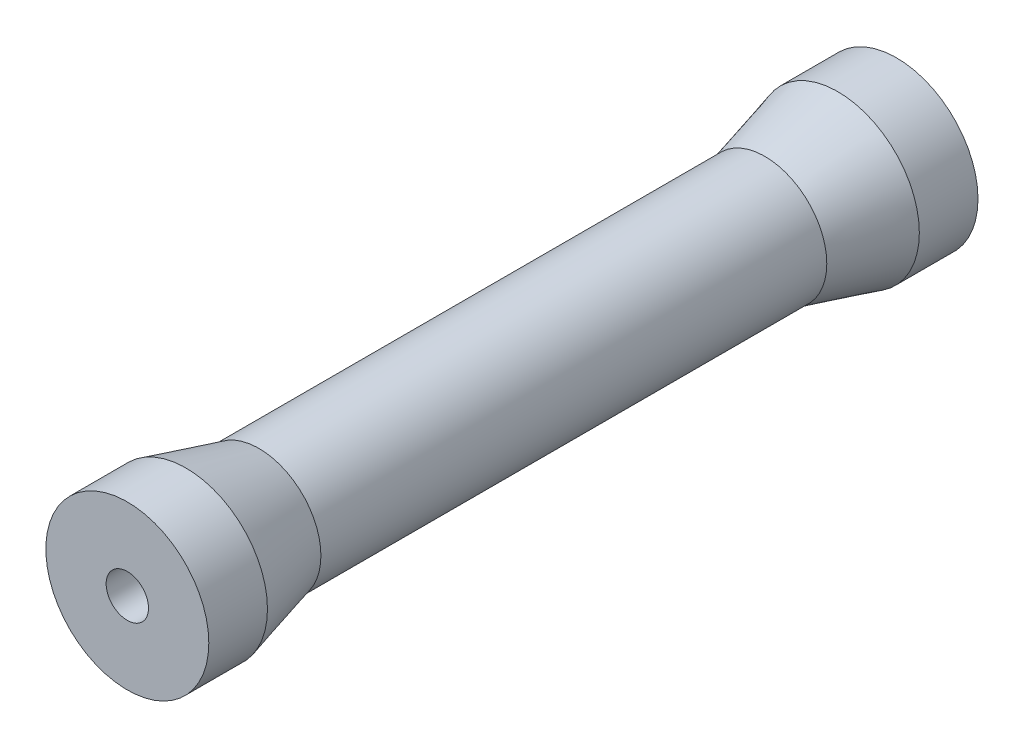
from build123d import *

# Parameters (mm, degrees)
SKETCH1_R           = 12.5
SKETCH1_R_2         = 3.25
BOSS_EXTRUDE1_DEPTH = 59


with BuildPart() as part:
    # Sketch1 → Boss-Extrude1 (new, symmetric)
    with BuildSketch(Plane.XY):
        Circle(SKETCH1_R)
        Circle(SKETCH1_R_2, mode=Mode.SUBTRACT)
    extrude(amount=BOSS_EXTRUDE1_DEPTH, both=True)

    # Sketch3 → Cut-Revolve1 (revolve, cut)
    with BuildSketch(Plane(origin=(0, 0, 0), x_dir=(1, 0, 0), z_dir=(0, 1, 0))):
        Polygon((12.5, -50), (12.5, 50), (9.5, 38.803847577), (9.5, -38.803847577), align=None)
    revolve(axis=Axis((0, 0, 0), (0, 0, -1)), mode=Mode.SUBTRACT)


solid = part.part
